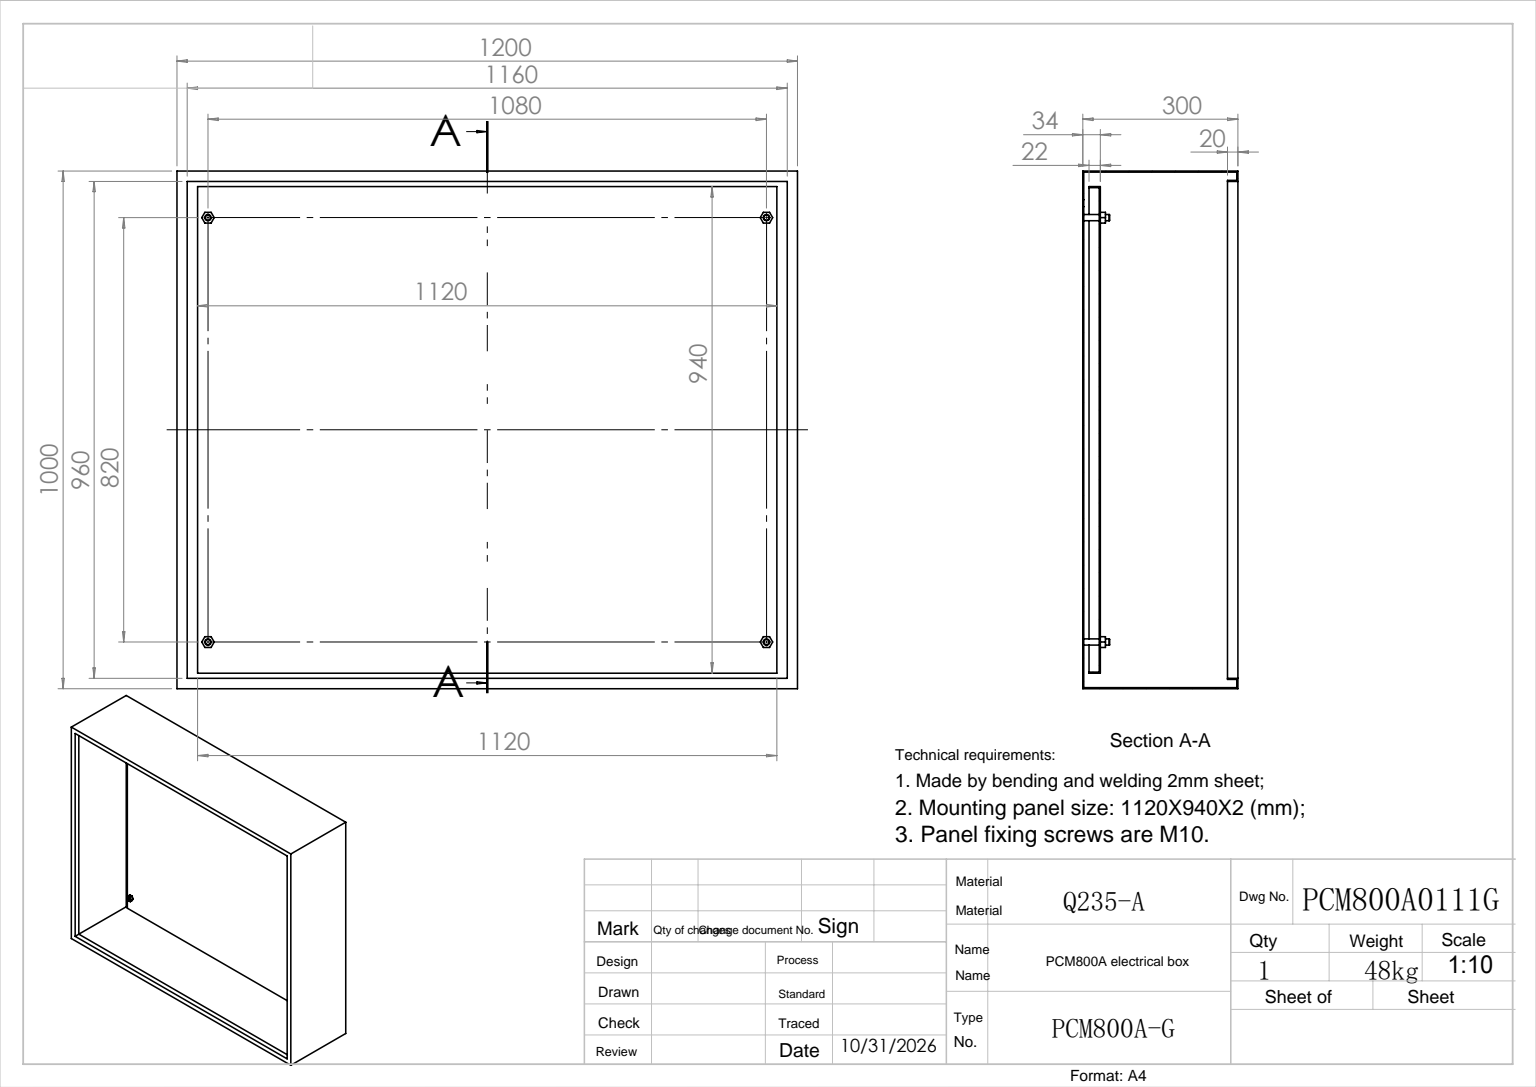
from build123d import *

# Parameters (mm, degrees)
SKETCH_1_W                     = 1200
SKETCH_1_H                     = 1000
EXTRUDE_1_DEPTH                = 300
SHELL_1_T                      = -2
SKETCH_2_R                     = 7
CUT_EXTRUDE_1_DEPTH            = 1591.221368238
PATTERN_LINEAR_1_COUNT         = 3
PATTERN_LINEAR_1_PITCH         = 388
PATTERN_LINEAR_2_COUNT         = 3
PATTERN_LINEAR_2_PITCH         = 538
SKETCH_3_W                     = 1200
SKETCH_3_H                     = 1000
SKETCH_3_W_2                   = 1160
SKETCH_3_H_2                   = 960
EXTRUDE_2_DEPTH                = 2
SKETCH_4_W                     = 1164
SKETCH_4_H                     = 964
SKETCH_4_W_2                   = 1160
SKETCH_4_H_2                   = 960
EXTRUDE_3_DEPTH                = 20
EXTRUDE_START                  = 30
SKETCH_5_W                     = 1120
SKETCH_5_H                     = 940
EXTRUDE_4_DEPTH                = 2
SKETCH_6_W                     = 1120
SKETCH_6_H                     = 940
SKETCH_6_W_2                   = 1116
SKETCH_6_H_2                   = 936
EXTRUDE_5_DEPTH                = 22
SKETCH_8_R                     = 6
EXTRUDE_6_DEPTH                = 50
FILLET_1_R                     = 1
EXTRUDE_7_DEPTH                = 10
PATTERN_LINEAR_4_COUNT         = 2
PATTERN_LINEAR_4_PITCH         = 1080
PATTERN_LINEAR_4_COUNT_DIR2    = 2
PATTERN_LINEAR_4_PITCH_DIR2    = 820
FILLET_1_OF_PATTERN_LINEAR_4_R = 1


with BuildPart() as part:
    # 草图1 → 凸台-拉伸1 (new body)
    with BuildSketch(Plane.XY):
        with Locations((600, -500)):
            Rectangle(SKETCH_1_W, SKETCH_1_H)
    extrude(amount=EXTRUDE_1_DEPTH)

    # 抽壳1
    shell_1_openings = [part.faces().sort_by_distance(p)[0] for p in [
        (600, -500, 300),
    ]]
    offset(amount=SHELL_1_T, openings=shell_1_openings, kind=Kind.INTERSECTION)

    # 草图2 → 切除-拉伸1 (cut, through all)
    with BuildSketch(Plane.XY.offset(2)):
        with Locations((60, -62)):
            Circle(SKETCH_2_R)
    cut_extrude_1 = extrude(amount=-CUT_EXTRUDE_1_DEPTH, mode=Mode.SUBTRACT)

    # 阵列(线性)1: 切除-拉伸1 ×3
    with Locations(*[(0, -i * PATTERN_LINEAR_1_PITCH, 0) for i in range(1, PATTERN_LINEAR_1_COUNT)]):
        add(cut_extrude_1, mode=Mode.SUBTRACT)

    # 阵列(线性)2: 切除-拉伸1 ×3
    with Locations(*[(i * PATTERN_LINEAR_2_PITCH, 0, 0) for i in range(1, PATTERN_LINEAR_2_COUNT)]):
        add(cut_extrude_1, mode=Mode.SUBTRACT)

    # 草图3 → 凸台-拉伸2 (add)
    with BuildSketch(Plane.XY.offset(300)):
        with Locations((600, -500)):
            Rectangle(SKETCH_3_W, SKETCH_3_H)
        with Locations((600, -500)):
            Rectangle(SKETCH_3_W_2, SKETCH_3_H_2, mode=Mode.SUBTRACT)
    extrude(amount=-EXTRUDE_2_DEPTH)

    # 草图4 → 凸台-拉伸3 (add)
    with BuildSketch(Plane.XY.offset(300)):
        with Locations((600, -500)):
            Rectangle(SKETCH_4_W, SKETCH_4_H)
        with Locations((600, -500)):
            Rectangle(SKETCH_4_W_2, SKETCH_4_H_2, mode=Mode.SUBTRACT)
    extrude(amount=-EXTRUDE_3_DEPTH)



with BuildPart() as body_2:
    # 草图5 → 凸台-拉伸4 (new body)
    with BuildSketch(Plane.XY.offset(2).offset(EXTRUDE_START)):
        with Locations((600, -500)):
            Rectangle(SKETCH_5_W, SKETCH_5_H)
    extrude(amount=EXTRUDE_4_DEPTH)

    # 草图6 → 凸台-拉伸5 (add)
    with BuildSketch(Plane.XY.offset(34)):
        with Locations((600, -500)):
            Rectangle(SKETCH_6_W, SKETCH_6_H)
        with Locations((600, -500)):
            Rectangle(SKETCH_6_W_2, SKETCH_6_H_2, mode=Mode.SUBTRACT)
    extrude(amount=-EXTRUDE_5_DEPTH)


with BuildPart() as part_1:
    add(part.part)

    add(body_2.part)  # 凸台-拉伸6 merges body 2
    # 草图8 → 凸台-拉伸6 (add)
    with BuildSketch(Plane.XY.offset(2)):
        with Locations((60, -90)):
            Circle(SKETCH_8_R)
    extrude_6 = extrude(amount=EXTRUDE_6_DEPTH)

    # 圆角1
    fillet_1_edges = [part_1.edges().sort_by_distance(p)[0] for p in [
        (54, -90, 52),
    ]]
    fillet(fillet_1_edges, radius=FILLET_1_R)

    # 草图9 → 凸台-拉伸7 (add)
    with BuildSketch(Plane.XY.offset(34)):
        Polygon((66, -79.607695155), (54, -79.607695155), (48, -90), (54, -100.392304845), (66, -100.392304845), (72, -90), align=None)
    extrude_7 = extrude(amount=EXTRUDE_7_DEPTH)

    # 阵列(线性)4: 凸台-拉伸6, Extrude 7 2 × 2
    with Locations(*[(i * PATTERN_LINEAR_4_PITCH, -j * PATTERN_LINEAR_4_PITCH_DIR2, 0) for i in range(PATTERN_LINEAR_4_COUNT) for j in range(PATTERN_LINEAR_4_COUNT_DIR2) if (i, j) != (0, 0)]):
        add(extrude_6)
        add(extrude_7)

    # 圆角1 of 阵列(线性)4
    fillet_1_of_pattern_linear_4_edges = [part_1.edges().sort_by_distance(p)[0] for p in [
        (54, -910, 52),
        (1134, -90, 52),
        (1134, -910, 52),
    ]]
    fillet(fillet_1_of_pattern_linear_4_edges, radius=FILLET_1_OF_PATTERN_LINEAR_4_R)


solid = part_1.part
